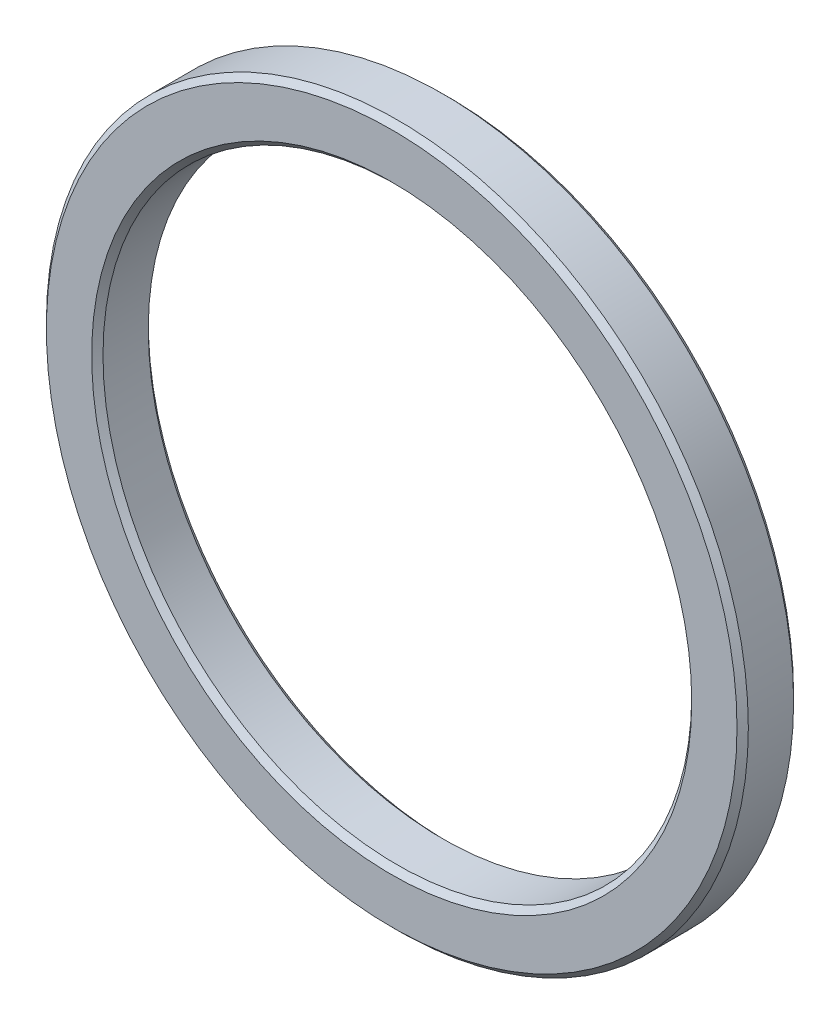
from build123d import *

# Parameters (mm, degrees)
SKETCH1_R           = 31
SKETCH1_R_2         = 26
BOSS_EXTRUDE1_DEPTH = 5
CHAMFER1_SIZE       = 0.5


with BuildPart() as part:
    # Sketch1 → Boss-Extrude1 (new body)
    with BuildSketch(Plane.XY):
        Circle(SKETCH1_R)
        Circle(SKETCH1_R_2, mode=Mode.SUBTRACT)
    extrude(amount=BOSS_EXTRUDE1_DEPTH)

    # Chamfer1
    chamfer1_edges = [part.edges().sort_by_distance(p)[0] for p in [
        (-31, 0, 0),
        (-31, 0, 5),
        (-26, 0, 0),
        (-26, 0, 5),
    ]]
    chamfer(chamfer1_edges, length=CHAMFER1_SIZE)


solid = part.part
